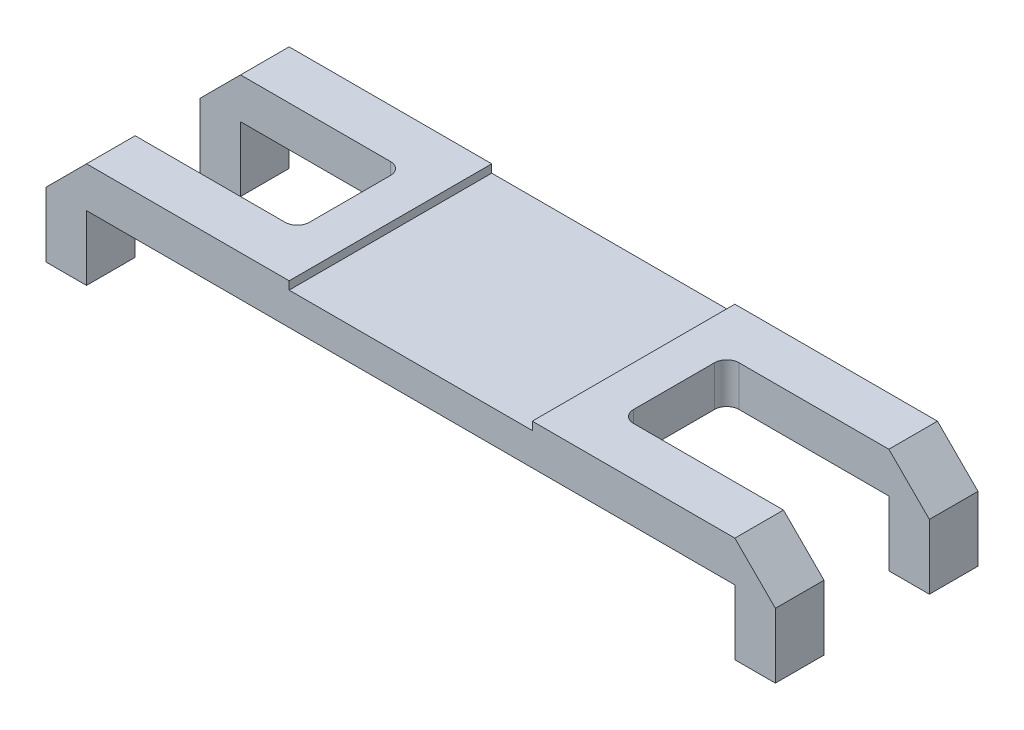
SolidWorks part; units mm, degrees
ref_plane "Front Plane" through (0, 0, 0) normal (0, 0, 1) x (1, 0, 0)
ref_plane "Top Plane" through (0, 0, 0) normal (0, 1, 0) x (1, 0, 0)
ref_plane "Right Plane" through (0, 0, 0) normal (1, 0, 0) x (0, 0, -1)
sketch "Sketch1" plane through (0, 0, 0) normal (0, 1, 0) x (1, 0, 0)
  line L1 (-90, 25) -> (90, 25)
  line L2 (-90, 25) -> (-90, -25)
  line L3 (-90, -25) -> (90, -25)
  line L4 (90, 25) -> (90, -25)
  line L5 (-90, 25) -> (90, -25) construction
  line L6 (-90, -25) -> (90, 25) construction
  point P0 (0, 0)
  dimension "D1" = 180
  dimension "D2" = 50
extrude "Boss-Extrude1" add sketch "Sketch1" along normal blind 10
sketch "Sketch2" plane through (0, 0, 0) normal (0, -1, 0) x (1, 0, 0)
  line L0 (-90, 25) -> (90, 25) construction
  line L1 (-90, -25) -> (-80, -25)
  line L2 (-90, -25) -> (-90, 25)
  line L3 (-90, 25) -> (-80, 25)
  line L4 (-80, -25) -> (-80, 25)
  line L6 (90, -25) -> (80, -25)
  line L7 (90, -25) -> (90, 25)
  line L8 (90, 25) -> (80, 25)
  line L9 (80, -25) -> (80, 25)
  dimension "D1" = 10
extrude "Boss-Extrude2" add sketch "Sketch2" along normal blind 16
sketch "Sketch3" plane through (0, 10, 0) normal (0, 1, 0) x (1, 0, 0)
  line L0 (-90, 25) -> (-90, -25) construction
  line L1 (-90, 13) -> (-40, 13)
  line L2 (-90, 13) -> (-90, -13)
  line L3 (-90, -13) -> (-40, -13)
  line L4 (-40, 13) -> (-40, -13)
  line L5 (90, 25) -> (-90, 25) construction
  line L6 (-90, -25) -> (90, -25) construction
  dimension "D1" = 12
  dimension "D2" = 12
  dimension "D3" = 50
extrude "Cut-Extrude1" cut sketch "Sketch3" against normal through all
mirror "Mirror1" about plane through (0, 0, 0) normal (1, 0, 0) of "Cut-Extrude1"
fillet "Fillet1" radius 3 4 edges at (40, 5, 13) (40, 5, -13) (-40, 5, 13) (-40, 5, -13)
chamfer "Chamfer1" distance 10 angle 45 4 edges at (90, 10, -19) (90, 10, 19) (-90, 10, 19) (-90, 10, -19)
sketch "Sketch4" plane through (0, 10, 0) normal (0, 1, 0) x (1, 0, 0)
  line L0 (-80, -25) -> (80, -25) construction
  line L1 (30, -25) -> (-30, -25)
  line L2 (30, -25) -> (30, 25)
  line L3 (30, 25) -> (-30, 25)
  line L4 (-30, -25) -> (-30, 25)
  line L5 (80, 25) -> (-80, 25) construction
  line L6 (0, 0) -> (0, 25) construction
  dimension "D1" = 60
extrude "Cut-Extrude2" cut sketch "Sketch4" against normal blind 2
